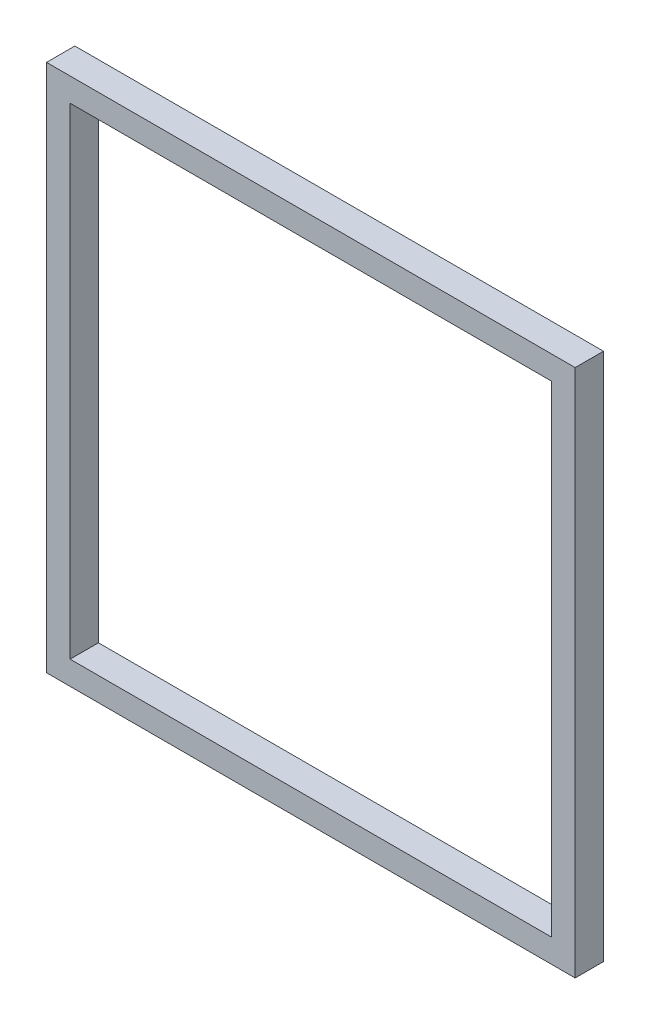
from build123d import *

# Parameters (mm, degrees)
SKETCH1_W           = 560
SKETCH1_H           = 560
SKETCH1_W_2         = 510
SKETCH1_H_2         = 510
BOSS_EXTRUDE1_DEPTH = 30


with BuildPart() as part:
    # Sketch1 → Boss-Extrude1 (new body)
    with BuildSketch(Plane.XY):
        with Locations((280, 280)):
            Rectangle(SKETCH1_W, SKETCH1_H)
        with Locations((280, 280)):
            Rectangle(SKETCH1_W_2, SKETCH1_H_2, mode=Mode.SUBTRACT)
    extrude(amount=BOSS_EXTRUDE1_DEPTH)


solid = part.part
